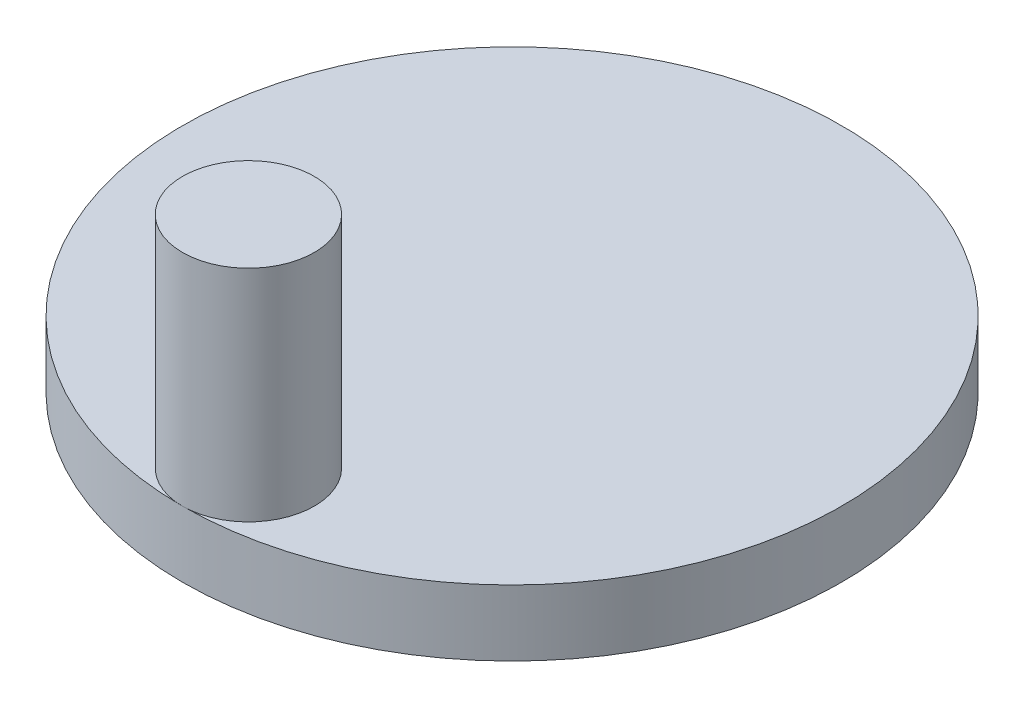
from build123d import *

# Parameters (mm, degrees)
SKETCH1_R           = 15
BOSS_EXTRUDE1_DEPTH = 3
SKETCH2_R           = 3
BOSS_EXTRUDE2_DEPTH = 10
SKETCH3_R           = 5
BOSS_EXTRUDE3_DEPTH = 2
SKETCH4_R           = 5
SKETCH4_W           = 4
SKETCH4_H           = 4
BOSS_EXTRUDE4_DEPTH = 5
SKETCH5_R           = 7.5
BOSS_EXTRUDE5_DEPTH = 2


with BuildPart() as part:
    # Sketch1 → Boss-Extrude1 (new body)
    with BuildSketch(Plane(origin=(0, 0, 0), x_dir=(1, 0, 0), z_dir=(0, 1, 0))):
        with Locations(Location((0, 0, 0), (0, 0, 270))):
            Circle(SKETCH1_R)
    extrude(amount=BOSS_EXTRUDE1_DEPTH)

    # Sketch2 → Boss-Extrude2 (add)
    with BuildSketch(Plane(origin=(0, 3, 0), x_dir=(1, 0, 0), z_dir=(0, 1, 0))):
        with Locations(Location((0, -12, 0), (0, 0, 270))):
            Circle(SKETCH2_R)
    extrude(amount=BOSS_EXTRUDE2_DEPTH)

    # Sketch3 → Boss-Extrude3 (add)
    with BuildSketch(Plane(origin=(0, 0, 0), x_dir=(-1, 0, 0), z_dir=(0, -1, 0))):
        with Locations(Location((0, 0, 0), (0, 0, 90))):
            Circle(SKETCH3_R)
    extrude(amount=BOSS_EXTRUDE3_DEPTH)

    # Sketch4 → Boss-Extrude4 (add)
    with BuildSketch(Plane(origin=(0, -2, 0), x_dir=(-1, 0, 0), z_dir=(0, -1, 0))):
        with Locations(Location((0, 0, 0), (0, 0, 90))):
            Circle(SKETCH4_R)
        Rectangle(SKETCH4_W, SKETCH4_H, mode=Mode.SUBTRACT)
    extrude(amount=BOSS_EXTRUDE4_DEPTH)

    # Sketch5 → Boss-Extrude5 (add)
    with BuildSketch(Plane(origin=(0, 0, 0), x_dir=(-1, 0, 0), z_dir=(0, -1, 0))):
        with Locations(Location((0, 0, 0), (0, 0, 270))):
            Circle(SKETCH5_R)
    extrude(amount=BOSS_EXTRUDE5_DEPTH)


solid = part.part
